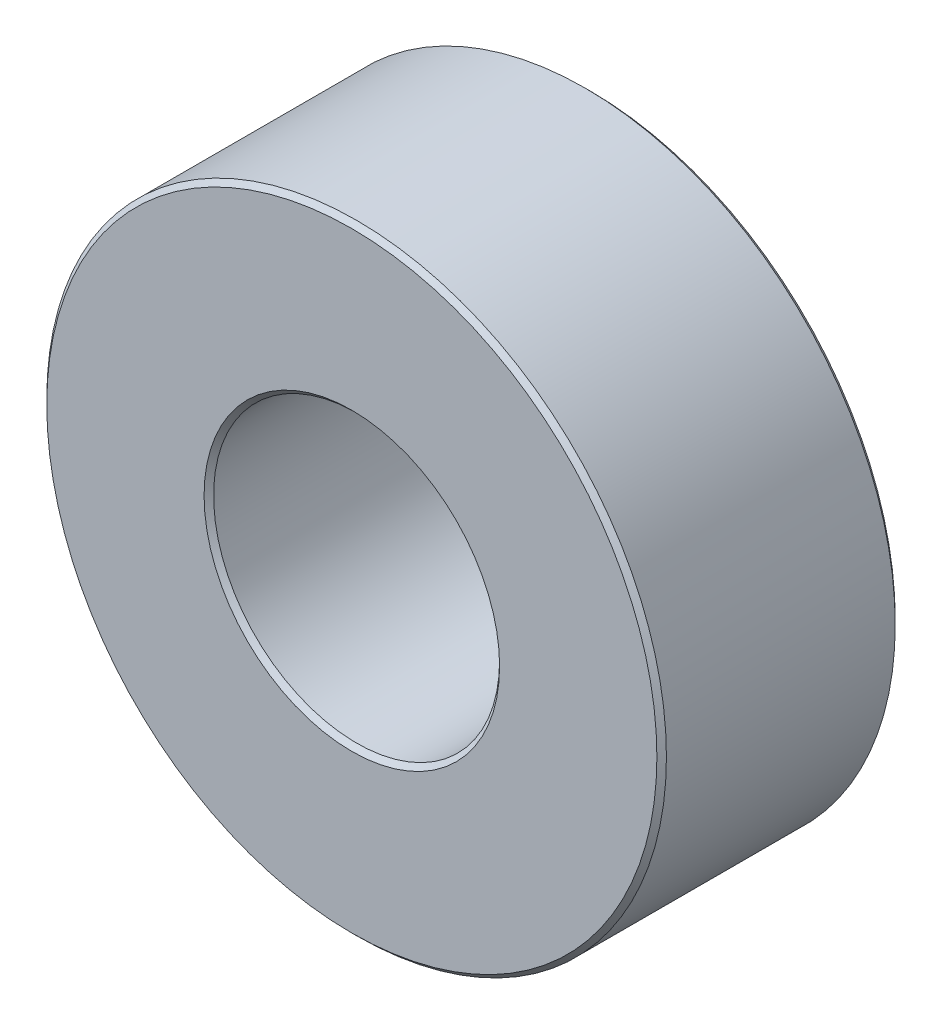
from build123d import *

# Parameters (mm, degrees)
SKETCH1_R           = 6.5
SKETCH1_R_2         = 3
BOSS_EXTRUDE1_DEPTH = 5
CHAMFER1_SIZE       = 0.1


with BuildPart() as part:
    # Sketch1 → Boss-Extrude1 (new body)
    with BuildSketch(Plane.XY):
        Circle(SKETCH1_R)
        Circle(SKETCH1_R_2, mode=Mode.SUBTRACT)
    extrude(amount=BOSS_EXTRUDE1_DEPTH)

    # Chamfer1
    chamfer1_edges = [part.edges().sort_by_distance(p)[0] for p in [
        (-6.5, 0, 0),
        (-6.5, 0, 5),
        (-3, 0, 0),
        (-3, 0, 5),
    ]]
    chamfer(chamfer1_edges, length=CHAMFER1_SIZE)


solid = part.part
